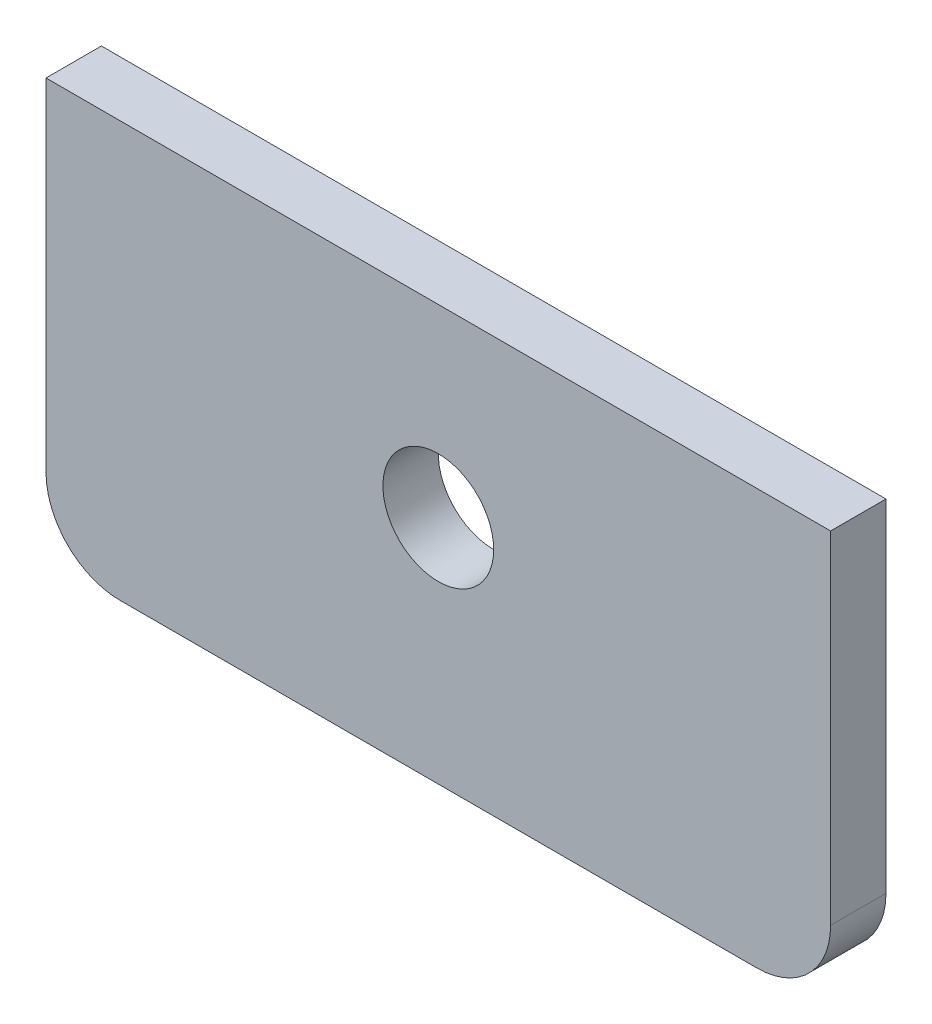
SolidWorks part; units mm, degrees
ref_plane "前视基准面" through (0, 0, 0) normal (0, 0, 1) x (1, 0, 0)
ref_plane "上视基准面" through (0, 0, 0) normal (0, 1, 0) x (1, 0, 0)
ref_plane "右视基准面" through (0, 0, 0) normal (1, 0, 0) x (0, 0, -1)
sketch "草图1" plane through (0, 0, 0) normal (0, 0, 1) x (1, 0, 0)
  line L0 (0, 0) -> (0, 10.7531) construction
  line L1 (-42.5, 22.5) -> (42.5, 22.5)
  line L2 (-42.5, 22.5) -> (-42.5, -14.5)
  line L3 (-34.5, -22.5) -> (34.5, -22.5)
  line L4 (42.5, 22.5) -> (42.5, -14.5)
  line L5 (-42.5, 22.5) -> (42.5, -22.5) construction
  line L6 (-42.5, -22.5) -> (42.5, 22.5) construction
  circle A0 centre (0, 2.5) radius 6
  arc A1 (34.5, -22.5) -> (42.5, -14.5) centre (34.5, -14.5) ccw
  arc A2 (-42.5, -14.5) -> (-34.5, -22.5) centre (-34.5, -14.5) ccw
  point P0 (0, 0)
  dimension "D3" = 12
  dimension "D4" = 20
  dimension "D5" = 8
  dimension "D1" = 85
  dimension "D2" = 45
extrude "凸台-拉伸1" add sketch "草图1" along normal blind 6
